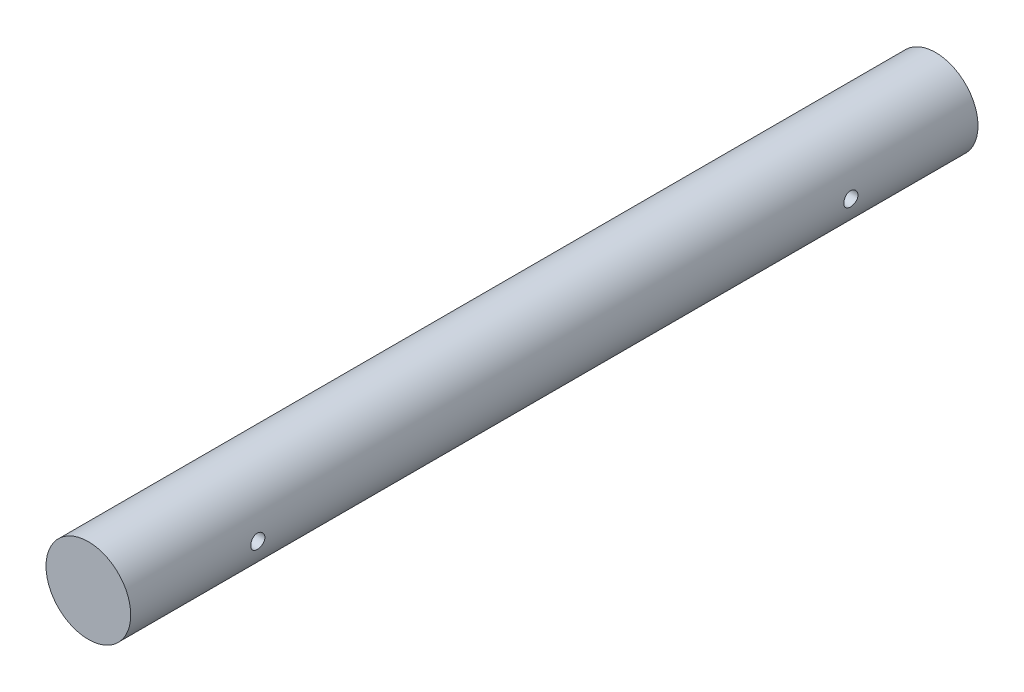
SolidWorks part; units mm, degrees
ref_plane "Front Plane" through (0, 0, 0) normal (0, 0, 1) x (1, 0, 0)
ref_plane "Top Plane" through (0, 0, 0) normal (0, 1, 0) x (1, 0, 0)
ref_plane "Right Plane" through (0, 0, 0) normal (1, 0, 0) x (0, 0, -1)
sketch "Sketch1" plane through (0, 0, 0) normal (0, 0, 1) x (1, 0, 0)
  circle A0 centre (-100, 71.3) radius 6
  dimension "D1" = 12
extrude "Boss-Extrude1" add sketch "Sketch1" against normal up to surface (60 mm away) and the other way up to surface (60 mm away) contours A0
ref_plane "Plane4" through (-100, 0, 0) normal (-1, 0, 0) x (0, 0, 1)
sketch "Sketch2" plane through (-100, 0, 0) normal (-1, 0, 0) x (0, 0, 1)
  line L0 (-60, 71.3) -> (60, 71.3) construction
  line L1 (-41, 93.3) -> (-41, -20) construction
  line L2 (0, -20) -> (0, 144.8897) construction
  line L3 (0, -24) -> (0, 5) construction
  circle A0 centre (-42, 71.3) radius 1
  circle A1 centre (42, 71.3) radius 1
  dimension "D1" = 2
extrude "Cut-Extrude1" cut sketch "Sketch2" against normal through all both and the other way through all
